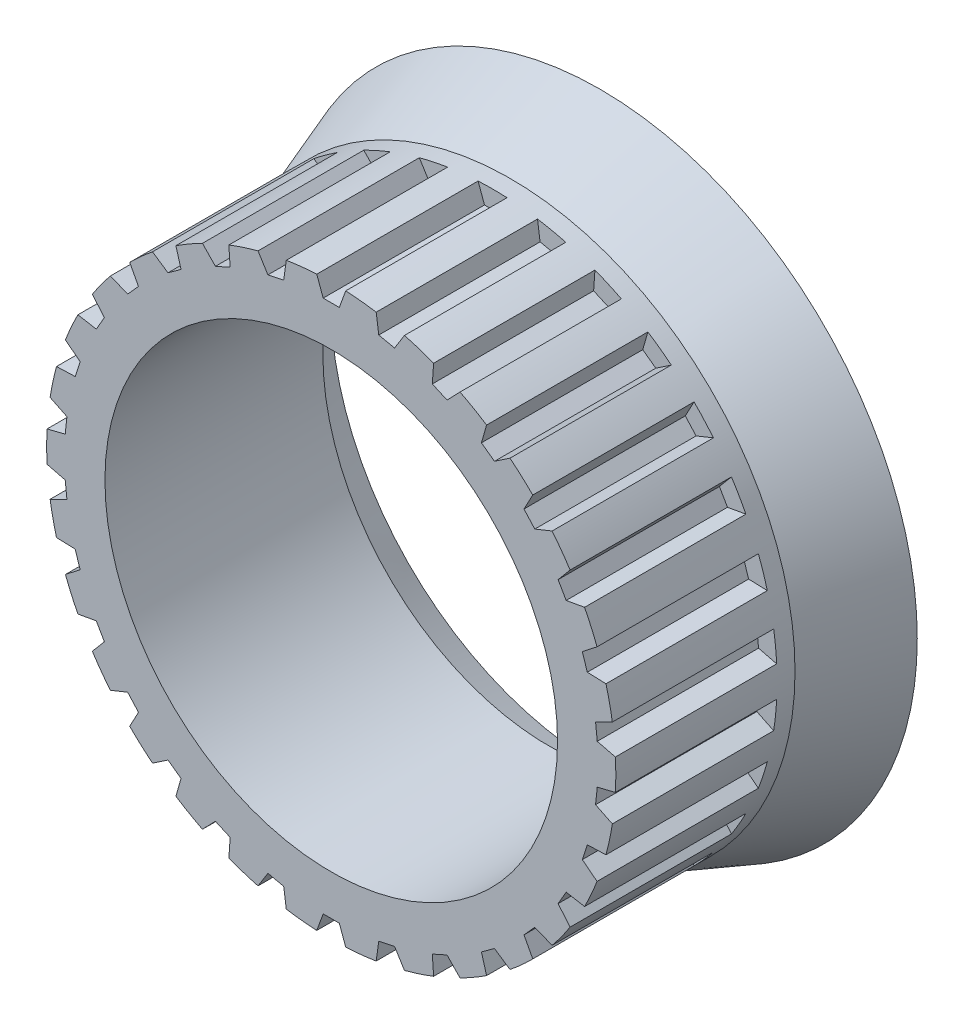
SolidWorks part; units mm, degrees
ref_plane "Front Plane" through (0, 0, 0) normal (0, 0, 1) x (1, 0, 0)
ref_plane "Top Plane" through (0, 0, 0) normal (0, 1, 0) x (1, 0, 0)
ref_plane "Right Plane" through (0, 0, 0) normal (1, 0, 0) x (0, 0, -1)
other "Configuration Table"
sketch "Sketch1" plane through (0, 0, 0) normal (1, 0, 0) x (0, 0, -1)
  line L0 (-16.883, 0) -> (9.8297, 0) construction
  line L1 (0, 31.75) -> (0, 0)
  line L3 (24.316, 28) -> (30, 30.0688)
  line L4 (30, 30.0688) -> (30, 35.3897)
  line L5 (30, 35.3897) -> (20, 31.75)
  line L6 (20, 31.75) -> (0, 31.75)
  line L7 (24.316, 28) -> (24.316, 0)
  line L8 (24.316, 0) -> (0, 0)
  dimension "D1" = 63.5
  dimension "D2" = 20
  dimension "D3" = 30
  dimension "D4" = 20
  dimension "D5" = 5
  dimension "D6" = 56
revolve "Revolve1" add sketch "Sketch1" angle 360 about L0
sketch "Sketch4" plane through (0, 0, 0) normal (0, 0, 1) x (1, 0, 0)
  circle A0 centre (0, 0) radius 8.2862
  point P0 (0, 0)
hole_wizard "M56 Tapped Hole1" positions "Sketch4" profile "Sketch5" tap size "M56" standard "GB"
sketch "Sketch5" plane through (0, 0, 0) normal (1, 0, 0) x (0, -1, 0)
  line L0 (0, 0) -> (0, 143.6717)
  line L1 (0, 143.6717) -> (25.25, 128.5)
  line L2 (25.25, 128.5) -> (25.25, 0)
  line L5 (25.25, 0) -> (0, 0)
  line L10 (0, 143.6717) -> (-25.25, 128.5) construction
  line L11 (0, -6.35) -> (0, 107.95) construction
  dimension "螺纹孔钻头直径" = 50.5
  dimension "螺纹孔钻头深度" = 128.5
  dimension "导头角度" = 118
cosmetic thread "Cosmetic Thread 1" parameters "D1"=112, "D2"=56
sketch "Sketch6" plane through (0, 0, 0) normal (0, 0, 1) x (1, 0, 0)
  line L0 (0, 41.3635) -> (0, -39.4114) construction
  line L1 (-1.613, -31.709) -> (-0.9, -29.75)
  line L2 (-0.9, -29.75) -> (0.9, -29.75)
  line L3 (0.9, -29.75) -> (1.613, -31.709)
  circle A0 centre (0, 0) radius 31.75
  circle M7 centre (0, 0) radius 31.75
  dimension "D1" = 63.5
  dimension "D2" = 1.8
  dimension "D3" = 29.75
  dimension "D4" = 40
extrude "Cut-Extrude1" cut sketch "Sketch6" against normal blind 18 contours L0 L2 L1 M7 | L2 L0 A0 L3
pattern_circular "CirPattern1" count 30 over 360 about axis through (0, 0, 0) along (0, 0, 1) of "Cut-Extrude1"
